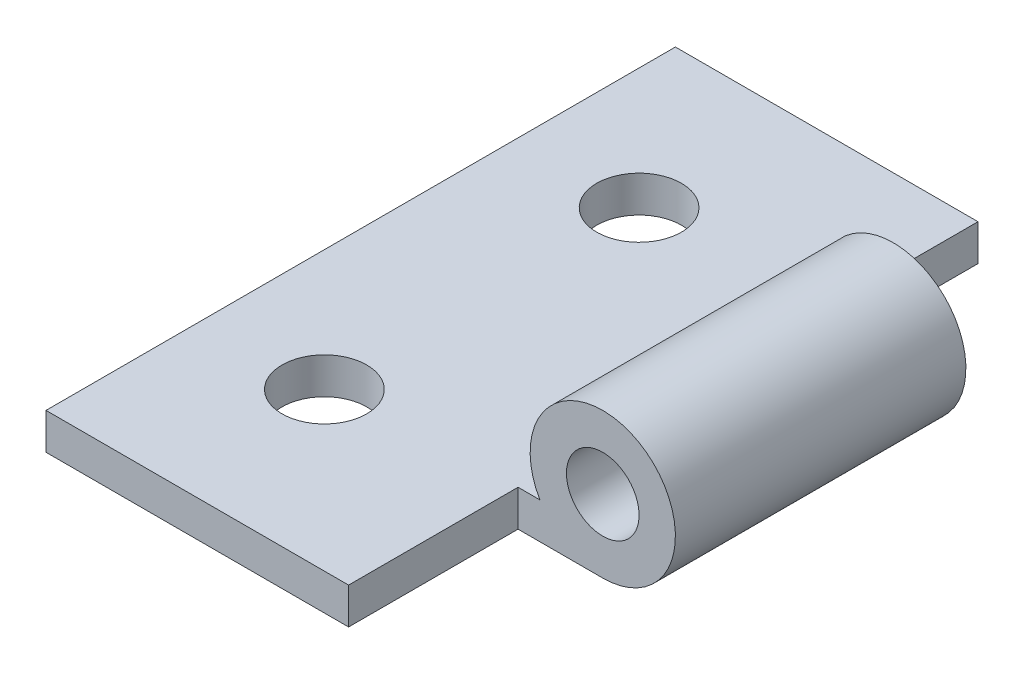
from build123d import *

# Parameters (mm, degrees)
SKETCH_1_R          = 1.5
EXTRUDE_1_DEPTH     = 13
CUT_EXTRUDE_3_DEPTH = 7
CUT_EXTRUDE_4_DEPTH = 7
SKETCH_3_R          = 1.75
CUT_EXTRUDE_2_DEPTH = 22.100947846


with BuildPart() as part:
    # 草图1 → 凸台-拉伸1 (new, symmetric)
    with BuildSketch(Plane.XY):
        with BuildLine():
            Line((-2.598076211, -1.5), (-16, -1.5))
            Line((-16, -1.5), (-16, -3))
            Line((-16, -3), (0, -3))
            ThreePointArc((0, -3), (1.5, 2.598076211), (-2.598076211, -1.5))
        make_face()
        with Locations(Location((0, 0, 0), (0, 0, 180))):
            Circle(SKETCH_1_R, mode=Mode.SUBTRACT)
    extrude(amount=EXTRUDE_1_DEPTH, both=True)

    # 草图2 → 切除-拉伸3 (cut)
    with BuildSketch(Plane.XY.offset(13)):
        with BuildLine():
            Line((-3.5, 0), (-3.5, -3))
            Line((-3.5, -3), (-1.802775638, -3))
            ThreePointArc((-1.802775638, -3), (3.046285831, 1.723410176), (-3.5, 0))
        make_face()
    extrude(amount=-CUT_EXTRUDE_3_DEPTH, mode=Mode.SUBTRACT)

    # 草图4 → 切除-拉伸4 (cut)
    with BuildSketch(Plane(origin=(0, 0, -13), x_dir=(-1, 0, 0), z_dir=(0, 0, -1))):
        with BuildLine():
            Line((3.5, -3), (3.5, 0))
            ThreePointArc((3.5, 0), (-3.046285831, 1.723410176), (1.802775638, -3))
            Line((1.802775638, -3), (3.5, -3))
        make_face()
    extrude(amount=-CUT_EXTRUDE_4_DEPTH, mode=Mode.SUBTRACT)

    # 草图3 → 切除-拉伸2 (cut, through all)
    with BuildSketch(Plane(origin=(0, -1.5, 0), x_dir=(1, 0, 0), z_dir=(0, 1, 0))):
        with Locations(Location((-11, 6.5, 0), (0, 0, 180))):
            Circle(SKETCH_3_R)
        with Locations((-11, -6.5)):
            Circle(SKETCH_3_R)
    extrude(amount=-CUT_EXTRUDE_2_DEPTH, mode=Mode.SUBTRACT)


solid = part.part
